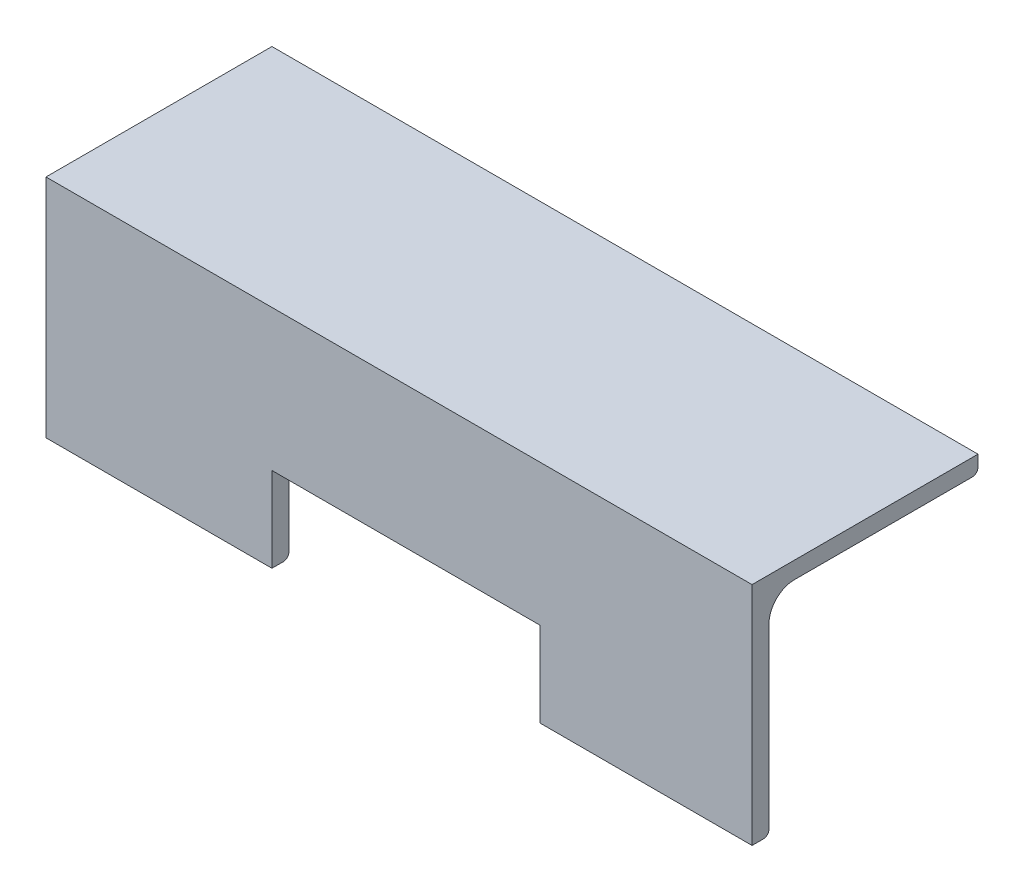
from build123d import *

# Parameters (mm, degrees)
HOT_ROLLED_EQUAL_ANGLE_STEEL_GB_T_9787_DEPTH = 250
SKETCH3_W                                    = 95
SKETCH3_H                                    = 49.519926073
CUT_EXTRUDE1_DEPTH                           = 10


with BuildPart() as part:
    # Sketch1 → hot-rolled equal angle steel (GB/T 9787-1988) 80×6(1) (new body)
    with BuildSketch(Plane(origin=(125, 0, 0), x_dir=(0, -1, 0), z_dir=(-1, 0, 0))):
        with BuildLine():
            Line((80, 0), (0, 0))
            Line((0, 0), (0, -80))
            Line((0, -80), (4, -80))
            ThreePointArc((4, -80), (5.414213562, -79.414213562), (6, -78))
            Line((6, -78), (6, -15))
            ThreePointArc((6, -15), (8.636038969, -8.636038969), (15, -6))
            Line((15, -6), (78, -6))
            ThreePointArc((78, -6), (79.414213562, -5.414213562), (80, -4))
            Line((80, -4), (80, 0))
        make_face()
    extrude(amount=HOT_ROLLED_EQUAL_ANGLE_STEEL_GB_T_9787_DEPTH)

    # Sketch3 → Cut-Extrude1 (cut)
    with BuildSketch(Plane(origin=(0, 0, -6), x_dir=(-1, 0, 0), z_dir=(0, 0, -1))):
        with Locations((-2.5, -74.759963037)):
            Rectangle(SKETCH3_W, SKETCH3_H)
    extrude(amount=-CUT_EXTRUDE1_DEPTH, mode=Mode.SUBTRACT)


solid = part.part
